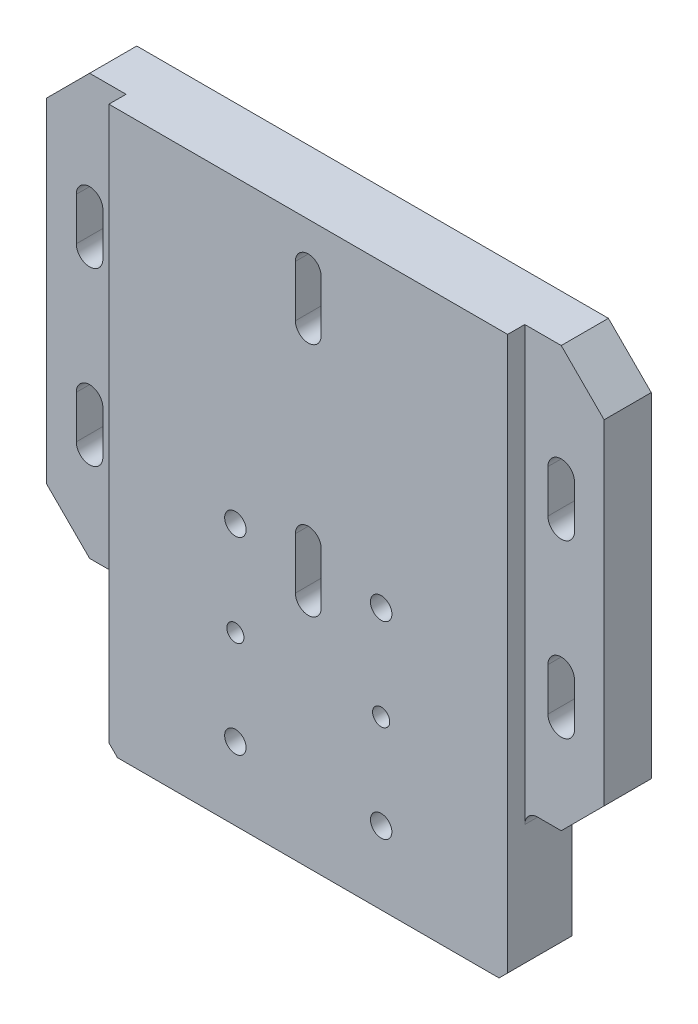
from build123d import *

# Parameters (mm, degrees)
SKETCH1_W               = 130
SKETCH1_H               = 131
EXTRUDE1_DEPTH          = 15
M6_TAPPED_HOLE1_D       = 5
EXTRUDE2_DEPTH          = 94.489304201
SKETCH5_W               = 18.5
SKETCH5_H               = 131
EXTRUDE3_DEPTH          = 4
CHAMFER1_SIZE           = 10
F_4_0_MM_DOWEL_HOLES1_D = 4
EXTRUDE4_DEPTH          = 94.489304201
EXTRUDE5_DEPTH          = 94.489304201
CHAMFER2_SIZE           = 10
CHAMFER3_SIZE           = 2


with BuildPart() as part:
    # Sketch1 → Extrude1 (new body)
    with BuildSketch(Plane.XY):
        Rectangle(SKETCH1_W, SKETCH1_H)
    extrude(amount=EXTRUDE1_DEPTH)

    # M6 Tapped Hole1 (through all)
    with Locations(Plane.XY.offset(15)):
        with Locations((17, -48.5), (-17, -48.5), (-17, -4.5), (17, -4.5)):
            Hole(M6_TAPPED_HOLE1_D / 2)

    # Sketch4 → Extrude2 (cut, through all)
    with BuildSketch(Plane.XY.offset(15)):
        with BuildLine():
            Line((-58.1, -10.5), (-58.1, -0.5))
            ThreePointArc((-58.1, -0.5), (-55, 2.6), (-51.9, -0.5))
            Line((-51.9, -0.5), (-51.9, -10.5))
            ThreePointArc((-51.9, -10.5), (-55, -13.6), (-58.1, -10.5))
        make_face()
        with BuildLine():
            Line((-58.1, 29.5), (-58.1, 39.5))
            ThreePointArc((-58.1, 39.5), (-55, 42.6), (-51.9, 39.5))
            Line((-51.9, 39.5), (-51.9, 29.5))
            ThreePointArc((-51.9, 29.5), (-55, 26.4), (-58.1, 29.5))
        make_face()
        with BuildLine():
            Line((51.9, -10.5), (51.9, -0.5))
            ThreePointArc((51.9, -0.5), (55, 2.6), (58.1, -0.5))
            Line((58.1, -0.5), (58.1, -10.5))
            ThreePointArc((58.1, -10.5), (55, -13.6), (51.9, -10.5))
        make_face()
        with BuildLine():
            Line((51.9, 29.5), (51.9, 39.5))
            ThreePointArc((51.9, 39.5), (55, 42.6), (58.1, 39.5))
            Line((58.1, 39.5), (58.1, 29.5))
            ThreePointArc((58.1, 29.5), (55, 26.4), (51.9, 29.5))
        make_face()
    extrude(amount=-EXTRUDE2_DEPTH, mode=Mode.SUBTRACT)

    # Sketch5 → Extrude3 (cut)
    with BuildSketch(Plane.XY.offset(15)):
        with Locations((-55.75, 0)):
            Rectangle(SKETCH5_W, SKETCH5_H)
        with Locations((55.75, 0)):
            Rectangle(SKETCH5_W, SKETCH5_H)
    extrude(amount=-EXTRUDE3_DEPTH, mode=Mode.SUBTRACT)

    # Chamfer1
    chamfer1_edges = [part.edges().sort_by_distance(p)[0] for p in [
        (-65, 65.5, 5.5),
        (65, 65.5, 5.5),
    ]]
    chamfer(chamfer1_edges, length=CHAMFER1_SIZE)

    # Ø4.0 mm Dowel Holes1 (through all)
    with Locations(Plane(origin=(0, 0, 0), x_dir=(-1, 0, 0), z_dir=(0, 0, -1))):
        with Locations((-17, -26.5), (17, -26.5)):
            Hole(F_4_0_MM_DOWEL_HOLES1_D / 2)

    # Sketch8 → Extrude4 (cut, through all)
    with BuildSketch(Plane.XY.offset(15)):
        with BuildLine():
            Line((-3, 43.5), (-3, 55.5))
            ThreePointArc((-3, 55.5), (0, 58.5), (3, 55.5))
            Line((3, 55.5), (3, 43.5))
            ThreePointArc((3, 43.5), (0, 40.5), (-3, 43.5))
        make_face()
        with BuildLine():
            Line((3, 0.5), (3, -11.5))
            ThreePointArc((3, -11.5), (0, -14.5), (-3, -11.5))
            Line((-3, -11.5), (-3, 0.5))
            ThreePointArc((-3, 0.5), (0, 3.5), (3, 0.5))
        make_face()
    extrude(amount=-EXTRUDE4_DEPTH, mode=Mode.SUBTRACT)

    # Sketch9 → Extrude5 (cut, through all)
    with BuildSketch(Plane.XY.offset(15)):
        with BuildLine():
            Line((-46.5, -65.5), (-65, -65.5))
            Line((-65, -65.5), (-65, -32.5))
            Line((-65, -32.5), (-49.5, -32.5))
            ThreePointArc((-49.5, -32.5), (-47.378679656, -33.378679656), (-46.5, -35.5))
            Line((-46.5, -35.5), (-46.5, -65.5))
        make_face()
        with BuildLine():
            Line((46.5, -65.5), (65, -65.5))
            Line((65, -65.5), (65, -32.5))
            Line((65, -32.5), (49.5, -32.5))
            ThreePointArc((49.5, -32.5), (47.378679656, -33.378679656), (46.5, -35.5))
            Line((46.5, -35.5), (46.5, -65.5))
        make_face()
    extrude(amount=-EXTRUDE5_DEPTH, mode=Mode.SUBTRACT)

    # Chamfer2
    chamfer2_edges = [part.edges().sort_by_distance(p)[0] for p in [
        (-65, -32.5, 5.5),
        (65, -32.5, 5.5),
    ]]
    chamfer(chamfer2_edges, length=CHAMFER2_SIZE)

    # Chamfer3
    chamfer3_edges = [part.edges().sort_by_distance(p)[0] for p in [
        (-46.5, -65.5, 7.5),
        (46.5, -65.5, 7.5),
    ]]
    chamfer(chamfer3_edges, length=CHAMFER3_SIZE)


solid = part.part
